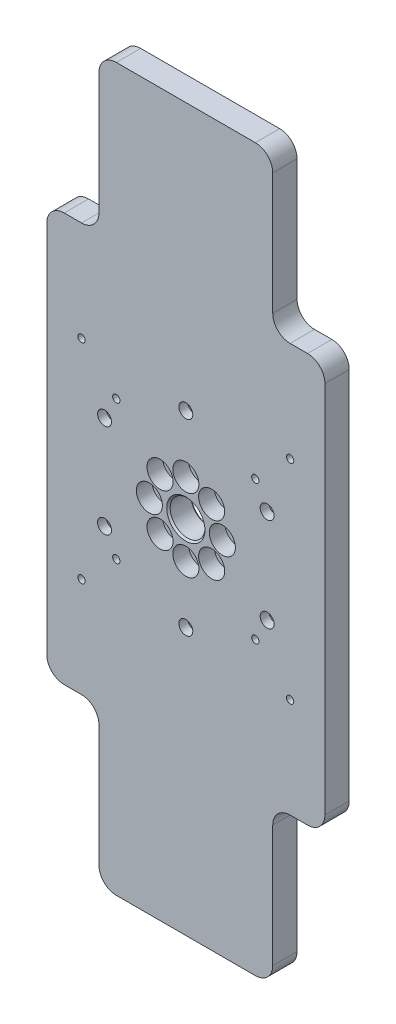
from build123d import *

# Parameters (mm, degrees)
SKETCH_1_R                = 10
EXTRUDE_1_DEPTH           = 7
HOLE_WIZARD_3_D           = 9
HOLE_WIZARD_3_CBORE_D     = 15
HOLE_WIZARD_3_CBORE_DEPTH = 9
PATTERN_CIRCULAR_1_COUNT  = 8
CHAMFER_1_SIZE            = 1
HOLE_WIZARD_6_0_6_1_D     = 6
SKETCH_14_R               = 4
CUT_EXTRUDE_1_DEPTH       = 5
HOLE_WIZARD_M5_1_D        = 4.2
PATTERN_CIRCULAR_2_COUNT  = 6
SKETCH_15_W               = 100
SKETCH_15_H               = 90
EXTRUDE_2_DEPTH           = 14
FILLET_1_R                = 10


with BuildPart() as part:
    # 草图1 → 凸台-拉伸1 (new, symmetric)
    with BuildSketch(Plane.XY):
        with BuildLine():
            Line((-70, 117.5), (70, 117.5))
            ThreePointArc((70, 117.5), (77.071067812, 114.571067812), (80, 107.5))
            Line((80, 107.5), (80, -107.5))
            ThreePointArc((80, -107.5), (77.071067812, -114.571067812), (70, -117.5))
            Line((70, -117.5), (-70, -117.5))
            ThreePointArc((-70, -117.5), (-77.071067812, -114.571067812), (-80, -107.5))
            Line((-80, -107.5), (-80, 107.5))
            ThreePointArc((-80, 107.5), (-77.071067812, 114.571067812), (-70, 117.5))
        make_face()
        Circle(SKETCH_1_R, mode=Mode.SUBTRACT)
    extrude(amount=EXTRUDE_1_DEPTH, both=True)

    # 打孔尺寸(%根据)内六角圆柱头螺钉的类型3 (through all)
    with Locations(Plane.XY.offset(7)):
        with Locations((0, 21)):
            hole_wizard_3 = CounterBoreHole(HOLE_WIZARD_3_D / 2, HOLE_WIZARD_3_CBORE_D / 2, HOLE_WIZARD_3_CBORE_DEPTH)

    # 阵列(圆周)1: 打孔尺寸(%根据)内六角圆柱头螺钉的类型3 ×8 about axis
    pattern_circular_1_axis = Axis((0, 0, 0), (0, 0, 1))
    for i in range(1, PATTERN_CIRCULAR_1_COUNT):
        add(hole_wizard_3.rotate(pattern_circular_1_axis, i * 360 / PATTERN_CIRCULAR_1_COUNT), mode=Mode.SUBTRACT)

    # 倒角1
    chamfer_1_edges = [part.edges().sort_by_distance(p)[0] for p in [
        (-10, 0, -7),
        (-10, 0, 7),
    ]]
    chamfer(chamfer_1_edges, length=CHAMFER_1_SIZE)

    # Ø6.0 (6) 直径孔1 (through all)
    with Locations(Plane.XY.offset(7)):
        with Locations((0, 54)):
            hole_wizard_6_0_6_1 = Hole(HOLE_WIZARD_6_0_6_1_D / 2)

    # 草图14 → 切除-拉伸1 (cut)
    with BuildSketch(Plane.XY.offset(7)):
        with Locations((0, 54)):
            Circle(SKETCH_14_R)
    cut_extrude_1 = extrude(amount=-CUT_EXTRUDE_1_DEPTH, mode=Mode.SUBTRACT)

    # M5 螺纹孔1 (through all)
    with Locations(Plane.XY.offset(7)):
        with Locations((-60, 60), (-40, 40), (40, 40), (40, -40), (-40, -40), (-60, -60), (60, -60), (60, 60)):
            Hole(HOLE_WIZARD_M5_1_D / 2)

    # 阵列(圆周)2: Ø6.0 (6) 直径孔1, 切除-拉伸1 ×6 about axis
    pattern_circular_2_axis = Axis((0, 0, 0), (0, 0, 1))
    add([hole_wizard_6_0_6_1.rotate(pattern_circular_2_axis, i * 360 / PATTERN_CIRCULAR_2_COUNT) for i in range(1, PATTERN_CIRCULAR_2_COUNT)], mode=Mode.SUBTRACT)
    add([cut_extrude_1.rotate(pattern_circular_2_axis, i * 360 / PATTERN_CIRCULAR_2_COUNT) for i in range(1, PATTERN_CIRCULAR_2_COUNT)], mode=Mode.SUBTRACT)

    # 草图15 → 凸台-拉伸2 (add)
    with BuildSketch(Plane.XY.offset(7)):
        with Locations((0, 162.5)):
            Rectangle(SKETCH_15_W, SKETCH_15_H)
    extrude_2 = extrude(amount=-EXTRUDE_2_DEPTH)

    # 镜向1: 凸台-拉伸2 across plane
    add(extrude_2.mirror(Plane.ZX))

    # 圆角1
    fillet_1_edges = [part.edges().sort_by_distance(p)[0] for p in [
        (50, 117.5, 0),
        (50, 207.5, 0),
        (-50, 207.5, 0),
        (-50, 117.5, 0),
        (-50, -207.5, 0),
        (-50, -117.5, 0),
        (50, -117.5, 0),
        (50, -207.5, 0),
    ]]
    fillet(fillet_1_edges, radius=FILLET_1_R)


solid = part.part
